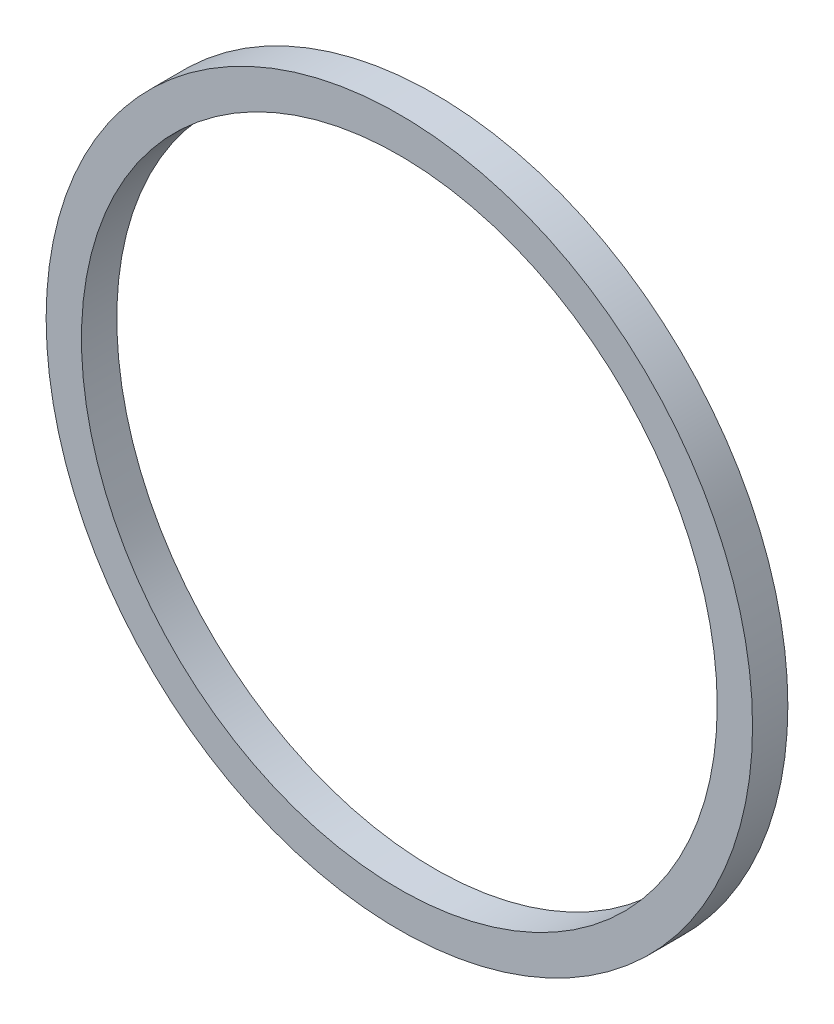
from build123d import *

# Parameters (mm, degrees)
SKETCH_1_R      = 30
SKETCH_1_R_2    = 27
EXTRUDE_1_DEPTH = 3


with BuildPart() as part:
    # 草图1 → 凸台-拉伸1 (new body)
    with BuildSketch(Plane.XY):
        Circle(SKETCH_1_R)
        Circle(SKETCH_1_R_2, mode=Mode.SUBTRACT)
    extrude(amount=EXTRUDE_1_DEPTH)


solid = part.part
